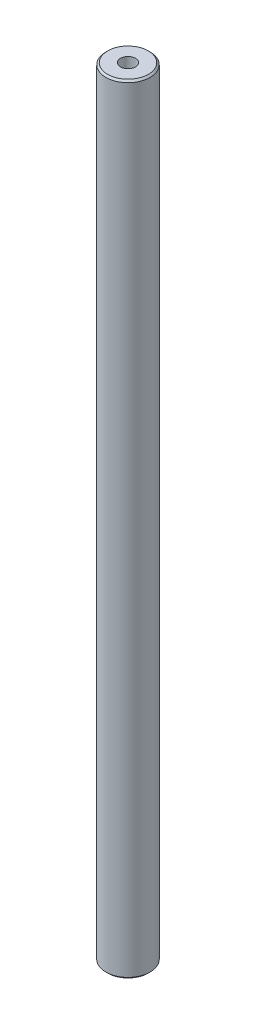
from build123d import *

# Parameters (mm, degrees)
SKETCH_1_R              = 12.5
EXTRUDE_1_DEPTH         = 440
CHAMFER_1_SIZE          = 1
HOLE_WIZARD_M10_1_D     = 8.5
HOLE_WIZARD_M10_1_DEPTH = 26.5
HOLE_WIZARD_M10_1_TIP   = 2.553657631


with BuildPart() as part:
    # 草图1 → 凸台-拉伸1 (new body)
    with BuildSketch(Plane(origin=(0, 0, 0), x_dir=(1, 0, 0), z_dir=(0, 1, 0))):
        with Locations(Location((0, 0, 0), (0, 0, 270))):
            Circle(SKETCH_1_R)
    extrude(amount=EXTRUDE_1_DEPTH)

    # 倒角1
    chamfer_1_edges = [part.edges().sort_by_distance(p)[0] for p in [
        (0, 0, -12.5),
        (0, 440, -12.5),
    ]]
    chamfer(chamfer_1_edges, length=CHAMFER_1_SIZE)

    # M10 螺纹孔1
    with Locations(Plane(origin=(0, 440, 0), x_dir=(1, 0, 0), z_dir=(0, 1, 0))):
        with Locations((0, 0)):
            Hole(HOLE_WIZARD_M10_1_D / 2, depth=HOLE_WIZARD_M10_1_DEPTH)
            with Locations((0, 0, -(HOLE_WIZARD_M10_1_DEPTH + HOLE_WIZARD_M10_1_TIP / 2))):  # 118° drill point
                Cone(0, HOLE_WIZARD_M10_1_D / 2, HOLE_WIZARD_M10_1_TIP, mode=Mode.SUBTRACT)


solid = part.part
